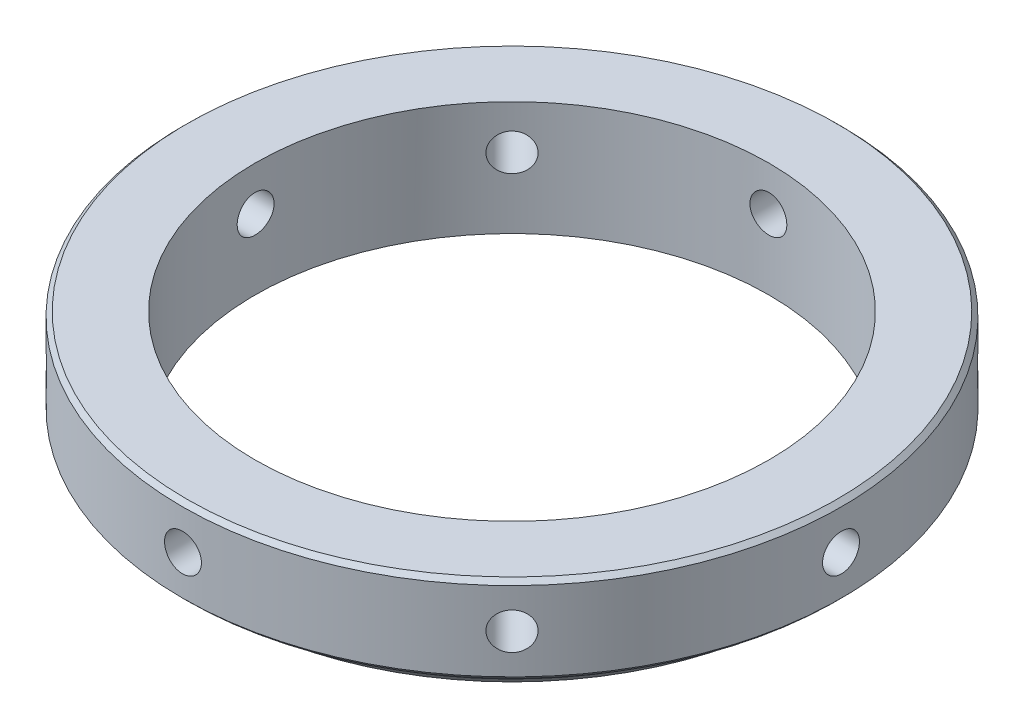
SolidWorks part; units mm, degrees
ref_plane "前视" through (0, 0, 0) normal (0, 0, 1) x (1, 0, 0)
ref_plane "上视" through (0, 0, 0) normal (0, 1, 0) x (1, 0, 0)
ref_plane "右视" through (0, 0, 0) normal (1, 0, 0) x (0, 0, -1)
sketch "草图1" plane through (0, 0, 0) normal (0, 1, 0) x (1, 0, 0)
  circle A0 centre (0, 0) radius 37.5
  circle A1 centre (0, 0) radius 29.25
  dimension "D1" = 75
  dimension "D2" = 58.5
extrude "凸台-拉伸1" add sketch "草图1" along normal mid plane 10
cosmetic thread "装饰螺纹线1" parameters "D2"=60
ref_plane "基准面1" through (0, 0, 40) normal (0, 0, 1) x (1, 0, 0)
hole_wizard "Ø4.2 (4.2) 直径孔1" positions "草图3" profile "草图2" hole size "Ø4.2" standard "Gb"
sketch "草图3" plane through (0, 0, 40) normal (0, 0, 1) x (1, 0, 0)
  point P0 (0, 0)
sketch "草图2" plane through (0, 0, 40) normal (1, 0, 0) x (0, -1, 0)
  line L0 (0, 0) -> (0, 16.2618)
  line L1 (0, 16.2618) -> (2.1, 15)
  line L2 (2.1, 15) -> (2.1, 0)
  line L5 (2.1, 0) -> (0, 0)
  line L10 (0, 16.2618) -> (-2.1, 15) construction
  line L11 (0, -6.35) -> (0, 107.95) construction
  dimension "孔直径" = 4.2
  dimension "孔深度" = 15
  dimension "导头角度" = 118
pattern_circular "阵列(圆周)1" count 8 over 360 about axis through (0, 5, 0) along (0, -1, 0) of "Ø4.2 (4.2) 直径孔1"
ref_plane "基准面2" through (34.6455, 0, 14.3506) normal (0.9239, 0, 0.3827) x (0.3827, 0, -0.9239)
chamfer "倒角1" distance 0.5 angle 45 2 edges at (0, -5, 37.5) (0, 5, 37.5)
sketch "草图6" plane through (0, -5, 0) normal (0, -1, 0) x (1, 0, 0)
  circle A0 centre (0, 0) radius 34.25
  circle A1 centre (0, 0) radius 29.25
  dimension "D1" = 58.5
  dimension "D2" = 68.5
extrude "凸台-拉伸2" add sketch "草图6" along normal blind 3
chamfer "倒角2" distance 1 angle 45 1 edges at (0, -8, -34.25)
